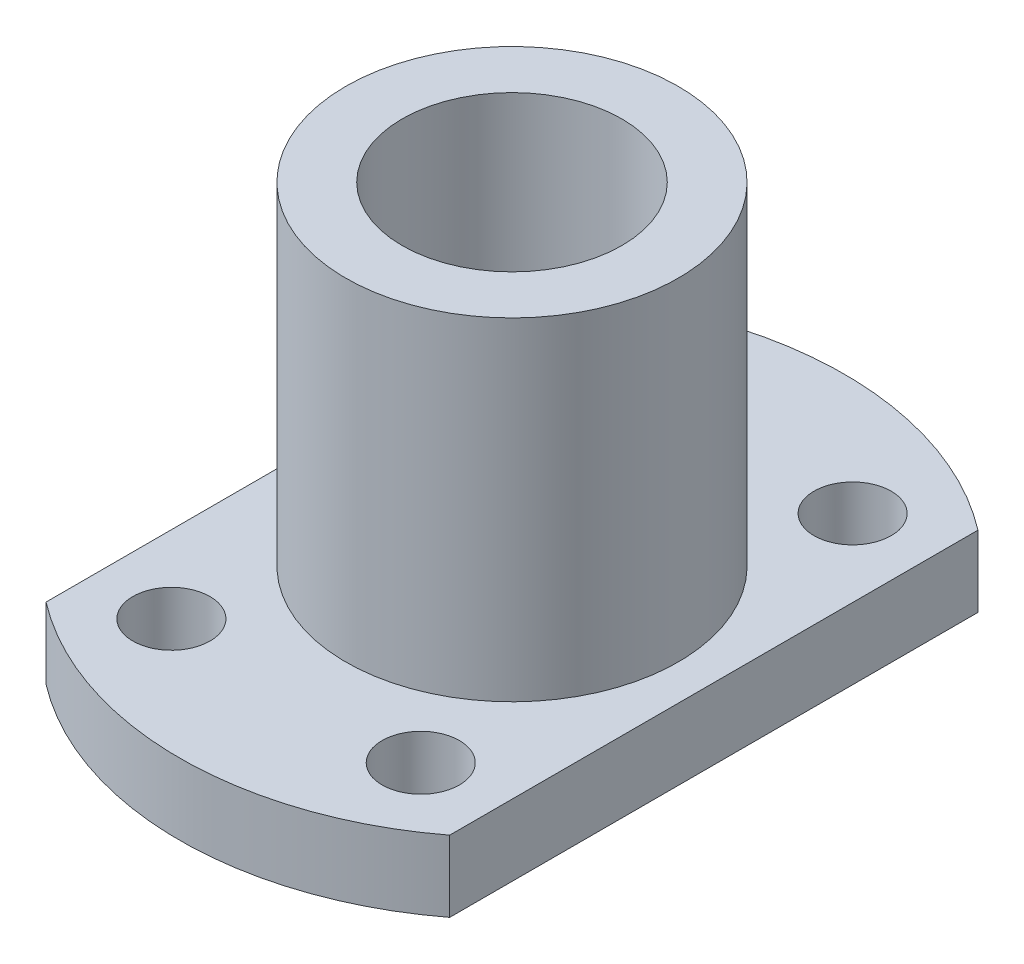
SolidWorks part; units mm, degrees
material "黄铜"
ref_plane "Front Plane" through (0, 0, 0) normal (0, 0, 1) x (1, 0, 0)
ref_plane "Top Plane" through (0, 0, 0) normal (0, 1, 0) x (1, 0, 0)
ref_plane "Right Plane" through (0, 0, 0) normal (1, 0, 0) x (0, 0, -1)
sketch "Sketch1" plane through (0, 0, 0) normal (0, 0, 1) x (1, 0, 0)
  line L0 (0, 0) -> (28, 0)
  line L1 (28, 0) -> (28, 6)
  line L2 (28, 6) -> (14, 6)
  line L3 (14, 6) -> (14, 34)
  line L4 (14, 34) -> (0, 34)
  line L5 (0, 34) -> (0, 0)
  dimension "D1" = 14
  dimension "D2" = 28
  dimension "D3" = 34
  dimension "D4" = 6
revolve "Revolve1" add sketch "Sketch1" angle 360 about L5
sketch "Sketch2" plane through (0, 0, 0) normal (0, -1, 0) x (1, 0, 0)
  line L1 (-17, 30) -> (17, 30)
  line L2 (-17, 30) -> (-17, -30)
  line L3 (-17, -30) -> (17, -30)
  line L4 (17, 30) -> (17, -30)
  dimension "D1" = 60
  dimension "D2" = 17
  dimension "D3" = 34
  dimension "D4" = 30
extrude "Cut-Extrude1" cut sketch "Sketch2" against normal blind 10 flip side to cut
hole_wizard "Ø6.5 (6.5) Diameter Hole1" positions "Sketch4" profile "Sketch3" hole size "Ø6.5" standard "GB"
sketch "Sketch4" plane through (0, 0, 0) normal (0, -1, 0) x (1, 0, 0)
  line L0 (0, 0) -> (21, 0) construction
  line L2 (-10.5, -18.1865) -> (10.5, 18.1865) construction
  line L5 (-10.5, 18.1865) -> (10.5, -18.1865) construction
  circle A0 centre (0, 0) radius 21 construction
  point P1 (-10.5, 18.1865)
  point P3 (10.5, 18.1865)
  point P5 (-10.5, -18.1865)
  point P7 (10.5, -18.1865)
  dimension "D3" = 42
  dimension "D1" = 60
  dimension "D2" = 60
sketch "Sketch3" plane through (-10.5, 0, 18.1865) normal (1, 0, 0) x (0, 0, -1)
  line L0 (0, 0) -> (0, 21.9528)
  line L1 (0, 21.9528) -> (3.25, 20)
  line L2 (3.25, 20) -> (3.25, 0)
  line L5 (3.25, 0) -> (0, 0)
  line L10 (0, 21.9528) -> (-3.25, 20) construction
  line L11 (0, -6.35) -> (0, 107.95) construction
  dimension "孔直径" = 6.5
  dimension "孔深度" = 20
  dimension "导头角度" = 118
hole_wizard "M20x1.5 Tapped Hole1" positions "Sketch6" profile "Sketch5" tap size "M20x1.5" standard "GB"
sketch "Sketch6" plane through (0, 0, 0) normal (0, -1, 0) x (1, 0, 0)
  point P0 (0, 0)
sketch "Sketch5" plane through (0, 0, 0) normal (1, 0, 0) x (0, 0, -1)
  line L0 (0, 0) -> (0, 50.058)
  line L1 (0, 50.058) -> (9.25, 44.5)
  line L2 (9.25, 44.5) -> (9.25, 0)
  line L5 (9.25, 0) -> (0, 0)
  line L10 (0, 50.058) -> (-9.25, 44.5) construction
  line L11 (0, -6.35) -> (0, 107.95) construction
  dimension "螺纹孔钻头直径" = 18.5
  dimension "螺纹孔钻头深度" = 44.5
  dimension "导头角度" = 118
cosmetic thread "孔螺蚊线1" parameters "D1"=40, "D2"=20
cosmetic thread "Cosmetic Thread1" parameters "D2"=20
